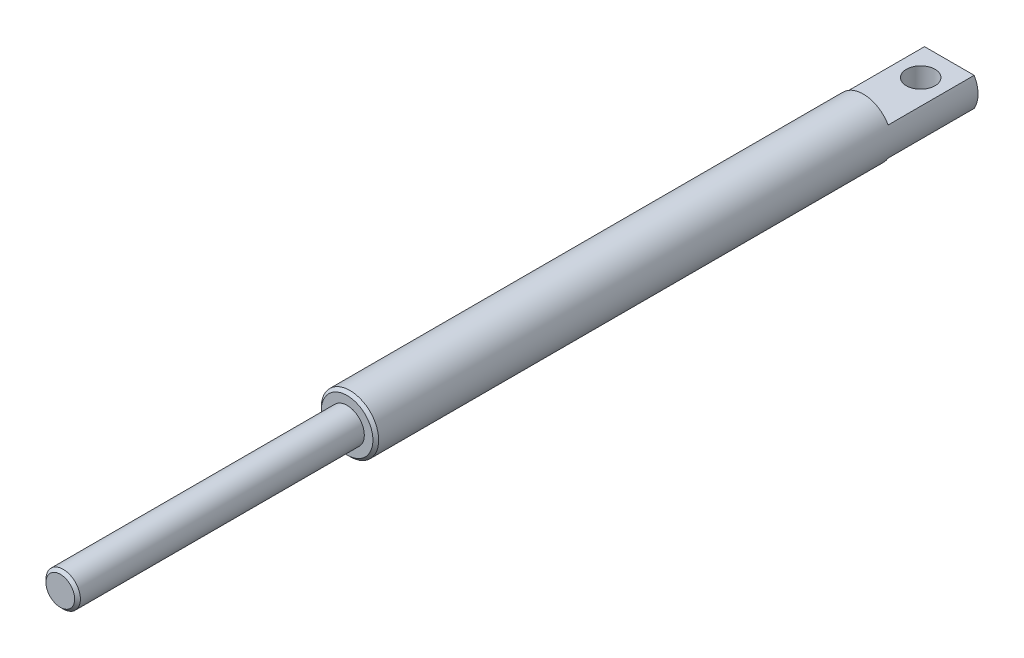
SolidWorks part; units mm, degrees
ref_plane "Front Plane" through (0, 0, 0) normal (0, 0, 1) x (1, 0, 0)
ref_plane "Top Plane" through (0, 0, 0) normal (0, 1, 0) x (1, 0, 0)
ref_plane "Right Plane" through (0, 0, 0) normal (1, 0, 0) x (0, 0, -1)
other "Configuration Table"
sketch "Sketch1" plane through (0, 0, 0) normal (0, 0, 1) x (1, 0, 0)
  circle A0 centre (0, 0) radius 10
  dimension "D1" = 20
extrude "Boss-Extrude1" add sketch "Sketch1" along normal blind 210
sketch "Sketch2" plane through (0, 0, 0) normal (0, 1, 0) x (1, 0, 0)
  line L0 (10, 0) -> (-10, 0) construction
  line L1 (-10, 0) -> (-10, -210) construction
  circle A0 centre (0, -10) radius 5
  dimension "D1" = 10
  dimension "D2" = 10
  dimension "D3" = 10
extrude "Cut-Extrude1" cut sketch "Sketch2" against normal through all both and the other way through all
sketch "Sketch3" plane through (0, 0, 0) normal (0, 0, -1) x (-1, 0, 0)
  line L1 (-18.4879, -5) -> (19.5242, -5)
  line L2 (-18.4879, -5) -> (-18.4879, -15.5085)
  line L3 (-18.4879, -15.5085) -> (19.5242, -15.5085)
  line L4 (19.5242, -5) -> (19.5242, -15.5085)
  line L5 (-15.2672, 14.8855) -> (17.4524, 14.8855)
  line L6 (-15.2672, 14.8855) -> (-15.2672, 5)
  line L7 (-15.2672, 5) -> (17.4524, 5)
  line L8 (17.4524, 14.8855) -> (17.4524, 5)
  dimension "D1" = 10
  dimension "D2" = 5
extrude "Cut-Extrude2" cut sketch "Sketch3" against normal blind 30 and the other way through all
sketch "Sketch4" plane through (0, 0, 210) normal (0, 0, 1) x (1, 0, 0)
  circle A0 centre (0, 0) radius 6
  dimension "D1" = 12
extrude "Boss-Extrude2" add sketch "Sketch4" along normal blind 100
cosmetic thread "Cosmetic Thread2" parameters "D1"=95, "D2"=11
chamfer "Chamfer1" distance 1 angle 45 2 edges at (6, 0, 310) (10, 0, 210)
